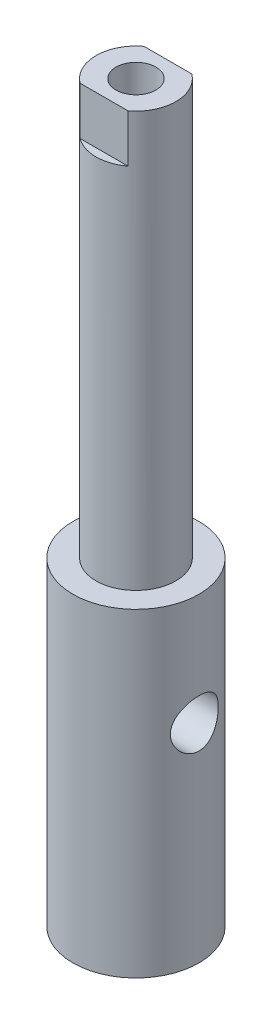
from build123d import *

# Parameters (mm, degrees)
SKETCH1_R               = 3.95
BOSS_EXTRUDE1_DEPTH     = 20
SKETCH2_R               = 2.5
BOSS_EXTRUDE2_DEPTH     = 26
SKETCH3_OUTSIDE_W       = 19.368
SKETCH3_OUTSIDE_H       = 19.368
SKETCH3_OUTSIDE_W_2     = 5.796030148
SKETCH3_OUTSIDE_H_2     = 4
CUT_EXTRUDE1_DEPTH      = 3
CUT_EXTRUDE2_DEPTH      = 47.337943416
CUT_EXTRUDE2_DEPTH_BACK = 47.337943416
SKETCH4_R               = 1.5
CUT_EXTRUDE3_START      = -1.5
SKETCH5_R               = 2
CUT_EXTRUDE3_DEPTH      = 10


with BuildPart() as part:
    # Sketch1 → Boss-Extrude1 (new body)
    with BuildSketch(Plane(origin=(0, 0, 0), x_dir=(1, 0, 0), z_dir=(0, 1, 0))):
        with Locations(Location((0, 0, 0), (0, 0, 270))):
            Circle(SKETCH1_R)
    extrude(amount=BOSS_EXTRUDE1_DEPTH)

    # Sketch2 → Boss-Extrude2 (add)
    with BuildSketch(Plane(origin=(0, 20, 0), x_dir=(1, 0, 0), z_dir=(0, 1, 0))):
        with Locations(Location((0, 0, 0), (0, 0, 90))):
            Circle(SKETCH2_R)
    extrude(amount=BOSS_EXTRUDE2_DEPTH)

    # Sketch3 outside → Cut-Extrude1 (cut)
    with BuildSketch(Plane(origin=(0, 46, 0), x_dir=(1, 0, 0), z_dir=(0, 1, 0))):
        Rectangle(SKETCH3_OUTSIDE_W, SKETCH3_OUTSIDE_H)
        Rectangle(SKETCH3_OUTSIDE_W_2, SKETCH3_OUTSIDE_H_2, mode=Mode.SUBTRACT)
    extrude(amount=-CUT_EXTRUDE1_DEPTH, mode=Mode.SUBTRACT)

    # Sketch4 → Cut-Extrude2 (cut, two sides: drawn at the far end of the back side and taken through both)
    with BuildSketch(Plane(origin=(0, 0, 0), x_dir=(0, 0, -1), z_dir=(1, 0, 0)).offset(-CUT_EXTRUDE2_DEPTH_BACK)):
        with Locations((0, 13)):
            Circle(SKETCH4_R)
    extrude(amount=CUT_EXTRUDE2_DEPTH + CUT_EXTRUDE2_DEPTH_BACK, mode=Mode.SUBTRACT)

    # Sketch5 → Cut-Extrude3 (cut)
    with BuildSketch(Plane(origin=(0, 0, 0), x_dir=(0, 0, -1), z_dir=(1, 0, 0)).offset(CUT_EXTRUDE3_START)):
        with Locations((0, 13)):
            Circle(SKETCH5_R)
    extrude(amount=-CUT_EXTRUDE3_DEPTH, mode=Mode.SUBTRACT)

    # Sketch6 → M3 Tapped Hole2 (revolve, cut)
    with BuildSketch(Plane(origin=(0, 46, 0), x_dir=(0, 0, 1), z_dir=(1, 0, 0))):
        Polygon((0, 0), (0, 8.251075774), (1.25, 7.5), (1.25, 0), align=None)
    revolve(axis=Axis((0, 52.35, 0), (0, -1, 0)), mode=Mode.SUBTRACT)


solid = part.part
